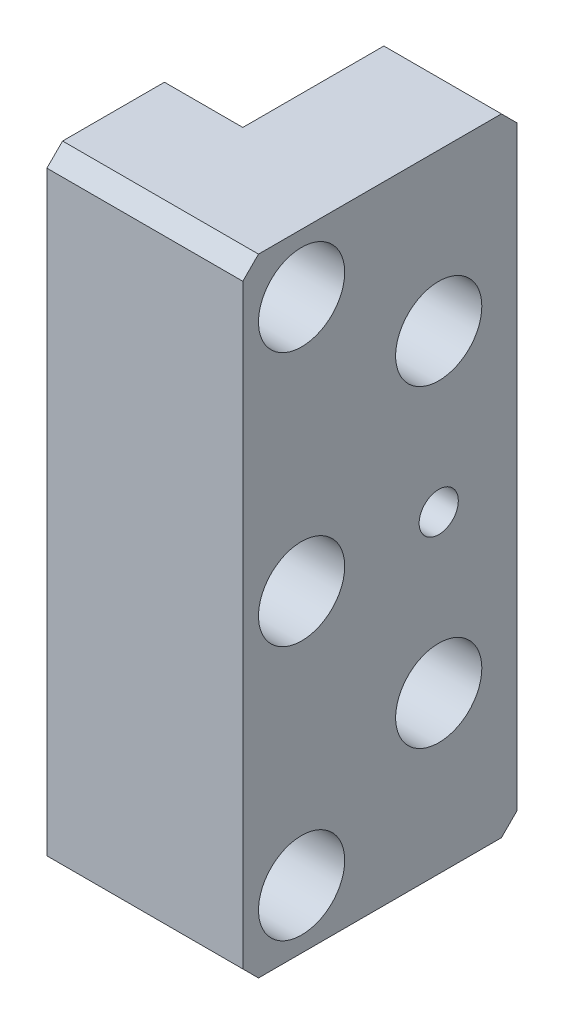
from build123d import *

# Parameters (mm, degrees)
EXTRUDE_1_DEPTH              = 40
CHAMFER_1_SIZE               = 2
HOLE_WIZARD_M6_1_D           = 6.6
HOLE_WIZARD_M6_1_CBORE_D     = 11
HOLE_WIZARD_M6_1_CBORE_DEPTH = 15
HOLE_WIZARD_M6_1_2_D         = 5
HOLE_WIZARD_M6_2_D           = 6.6
HOLE_WIZARD_M6_2_CBORE_D     = 11
HOLE_WIZARD_M6_2_CBORE_DEPTH = 8


with BuildPart() as part:
    # 草图1 → 凸台-拉伸1 (new, symmetric)
    with BuildSketch(Plane(origin=(0, 0, 0), x_dir=(1, 0, 0), z_dir=(0, 1, 0))):
        Polygon((0, 0), (25, 0), (25, 35), (10, 35), (10, 15), (0, 15), align=None)
    extrude(amount=EXTRUDE_1_DEPTH, both=True)

    # 倒角1
    chamfer_1_edges = [part.edges().sort_by_distance(p)[0] for p in [
        (17.5, 40, -35),
        (17.5, -40, -35),
        (12.5, -40, 0),
        (12.5, 40, 0),
    ]]
    chamfer(chamfer_1_edges, length=CHAMFER_1_SIZE)

    # Hole Wizard M6 _1 (through all)
    with Locations(Plane(origin=(25, 0, 0), x_dir=(0, 0, -1), z_dir=(1, 0, 0))):
        with Locations((7.5, 32.5), (7.5, 0), (7.5, -32.5)):
            CounterBoreHole(HOLE_WIZARD_M6_1_D / 2, HOLE_WIZARD_M6_1_CBORE_D / 2, HOLE_WIZARD_M6_1_CBORE_DEPTH)

    # Hole Wizard M6 _1 2 (through all)
    with Locations(Plane(origin=(25, 0, 0), x_dir=(0, 0, -1), z_dir=(1, 0, 0))):
        with Locations((25, 0)):
            Hole(HOLE_WIZARD_M6_1_2_D / 2)

    # M6 六角圆柱头螺钉的柱形沉头孔2 (through all)
    with Locations(Plane(origin=(25, 0, 0), x_dir=(0, 0, -1), z_dir=(1, 0, 0))):
        with Locations((25, 20), (25, -20)):
            CounterBoreHole(HOLE_WIZARD_M6_2_D / 2, HOLE_WIZARD_M6_2_CBORE_D / 2, HOLE_WIZARD_M6_2_CBORE_DEPTH)


solid = part.part
